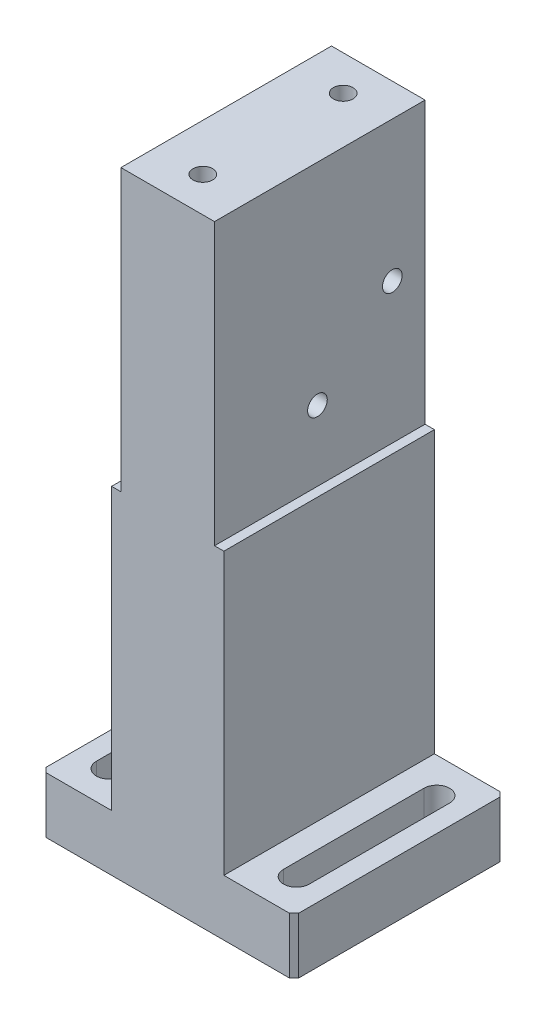
from build123d import *

# Parameters (mm, degrees)
BOSS_EXTRUDE1_DEPTH            = 45
SKETCH9_W                      = 2
SKETCH9_H                      = 60
CUT_EXTRUDE1_DEPTH             = 143.049287221
M5_TAPPED_HOLE2_D              = 4.2
F_5_5_5_5_DIAMETER_HOLE1_D     = 5.5
F_5_5_5_5_DIAMETER_HOLE1_DEPTH = 20
F_5_5_5_5_DIAMETER_HOLE1_TIP   = 1.652366702
CHAMFER1_SIZE                  = 1
M5_TAPPED_HOLE3_D              = 4.2
M5_TAPPED_HOLE3_DEPTH          = 14
M5_TAPPED_HOLE3_TIP            = 1.2618073
CUT_EXTRUDE2_REACH             = 144.049


with BuildPart() as part:
    # Sketch1 → Boss-Extrude1 (new body)
    with BuildSketch(Plane.XY):
        Polygon((27, 0), (-27, 0), (-27, 12), (-12, 12), (-12, 132), (12, 132), (12, 12), (27, 12), align=None)
    extrude(amount=BOSS_EXTRUDE1_DEPTH)

    # Sketch9 → Cut-Extrude1 (cut, through all)
    with BuildSketch(Plane.XY.offset(45)):
        with Locations((-11, 102)):
            Rectangle(SKETCH9_W, SKETCH9_H)
        with Locations((11, 102)):
            Rectangle(SKETCH9_W, SKETCH9_H)
    extrude(amount=-CUT_EXTRUDE1_DEPTH, mode=Mode.SUBTRACT)

    # M5 Tapped Hole2 (through all)
    with Locations(Plane(origin=(10, -0.235974088, -1.632115168), x_dir=(0, 0, -1), z_dir=(1, 0, 0))):
        with Locations((-8.632115168, 102.235974088), (-24.632115168, 87.235974088)):
            Hole(M5_TAPPED_HOLE2_D / 2)

    # Ø5.5 (5.5) Diameter Hole1
    with Locations(Plane(origin=(0, 12, 0), x_dir=(-1, 0, 0), z_dir=(0, 1, 0))):
        with Locations((20, 7.5), (20, 37.5), (-20, 37.5), (-20, 7.5)):
            Hole(F_5_5_5_5_DIAMETER_HOLE1_D / 2, depth=F_5_5_5_5_DIAMETER_HOLE1_DEPTH)
            with Locations((0, 0, -(F_5_5_5_5_DIAMETER_HOLE1_DEPTH + F_5_5_5_5_DIAMETER_HOLE1_TIP / 2))):  # 118° drill point
                Cone(0, F_5_5_5_5_DIAMETER_HOLE1_D / 2, F_5_5_5_5_DIAMETER_HOLE1_TIP, mode=Mode.SUBTRACT)

    # Chamfer1
    chamfer1_edges = [part.edges().sort_by_distance(p)[0] for p in [
        (27, 6, 45),
        (-27, 6, 0),
        (-27, 6, 45),
        (27, 6, 0),
    ]]
    chamfer(chamfer1_edges, length=CHAMFER1_SIZE)

    # M5 Tapped Hole3
    with Locations(Plane(origin=(0, 132, 0), x_dir=(-1, 0, 0), z_dir=(0, 1, 0))):
        with Locations((0, 37.5), (0, 7.5)):
            Hole(M5_TAPPED_HOLE3_D / 2, depth=M5_TAPPED_HOLE3_DEPTH)
            with Locations((0, 0, -(M5_TAPPED_HOLE3_DEPTH + M5_TAPPED_HOLE3_TIP / 2))):  # 118° drill point
                Cone(0, M5_TAPPED_HOLE3_D / 2, M5_TAPPED_HOLE3_TIP, mode=Mode.SUBTRACT)

    # Sketch12 → Cut-Extrude2 (cut, up to next)
    with BuildSketch(Plane.XZ, mode=Mode.PRIVATE) as cut_extrude2_sk1:
        with BuildLine():
            Line((-17.25, 37.5), (-17.25, 7.5))
            ThreePointArc((-17.25, 7.5), (-20, 4.75), (-22.75, 7.5))
            Line((-22.75, 7.5), (-22.75, 37.5))
            ThreePointArc((-22.75, 37.5), (-20, 40.25), (-17.25, 37.5))
        make_face()
    cut_extrude2_tool1 = extrude(cut_extrude2_sk1.sketch, amount=-CUT_EXTRUDE2_REACH, mode=Mode.PRIVATE) & part.part
    # Sketch12 → Cut-Extrude2 (cut, up to next)
    with BuildSketch(Plane.XZ, mode=Mode.PRIVATE) as cut_extrude2_sk2:
        with BuildLine():
            Line((22.75, 37.5), (22.75, 7.5))
            ThreePointArc((22.75, 7.5), (20, 4.75), (17.25, 7.5))
            Line((17.25, 7.5), (17.25, 37.5))
            ThreePointArc((17.25, 37.5), (20, 40.25), (22.75, 37.5))
        make_face()
    cut_extrude2_tool2 = extrude(cut_extrude2_sk2.sketch, amount=-CUT_EXTRUDE2_REACH, mode=Mode.PRIVATE) & part.part
    add(cut_extrude2_tool1.solids().sort_by_distance((-20, 0, 22.5))[0], mode=Mode.SUBTRACT)
    add(cut_extrude2_tool2.solids().sort_by_distance((20, 0, 22.5))[0], mode=Mode.SUBTRACT)


solid = part.part
